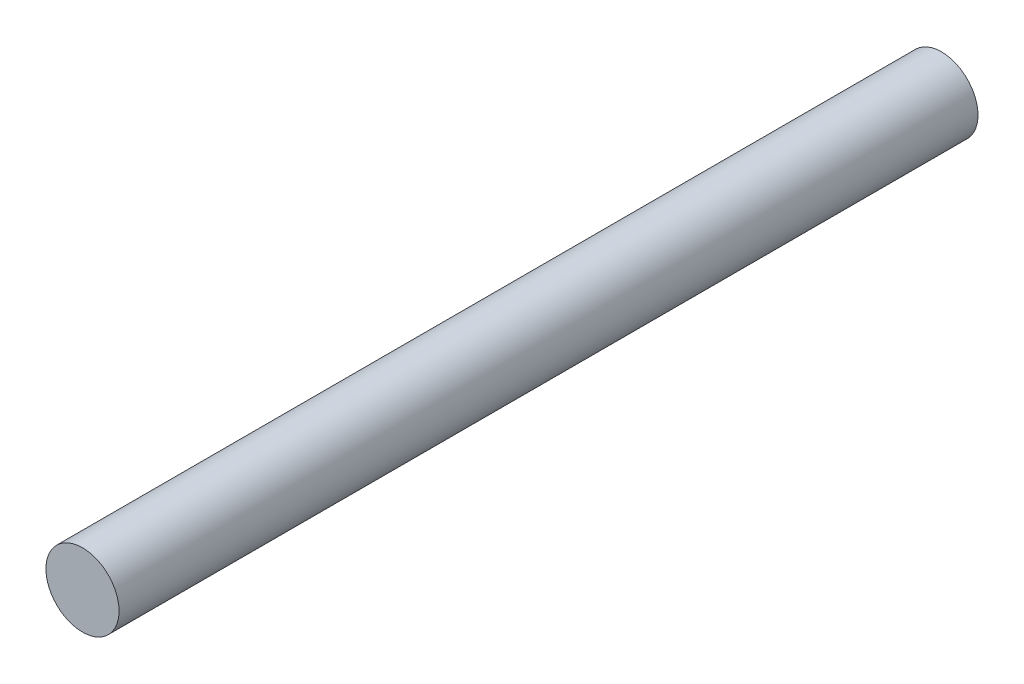
SolidWorks part; units mm, degrees
ref_plane "前视基准面" through (0, 0, 0) normal (0, 0, 1) x (1, 0, 0)
ref_plane "上视基准面" through (0, 0, 0) normal (0, 1, 0) x (1, 0, 0)
ref_plane "右视基准面" through (0, 0, 0) normal (1, 0, 0) x (0, 0, -1)
sketch "草图1" plane through (0, 0, 0) normal (0, 0, 1) x (1, 0, 0)
  circle A0 centre (0, 0) radius 2
  dimension "D1" = 4
extrude "凸台-拉伸1" add sketch "草图1" along normal blind 47
